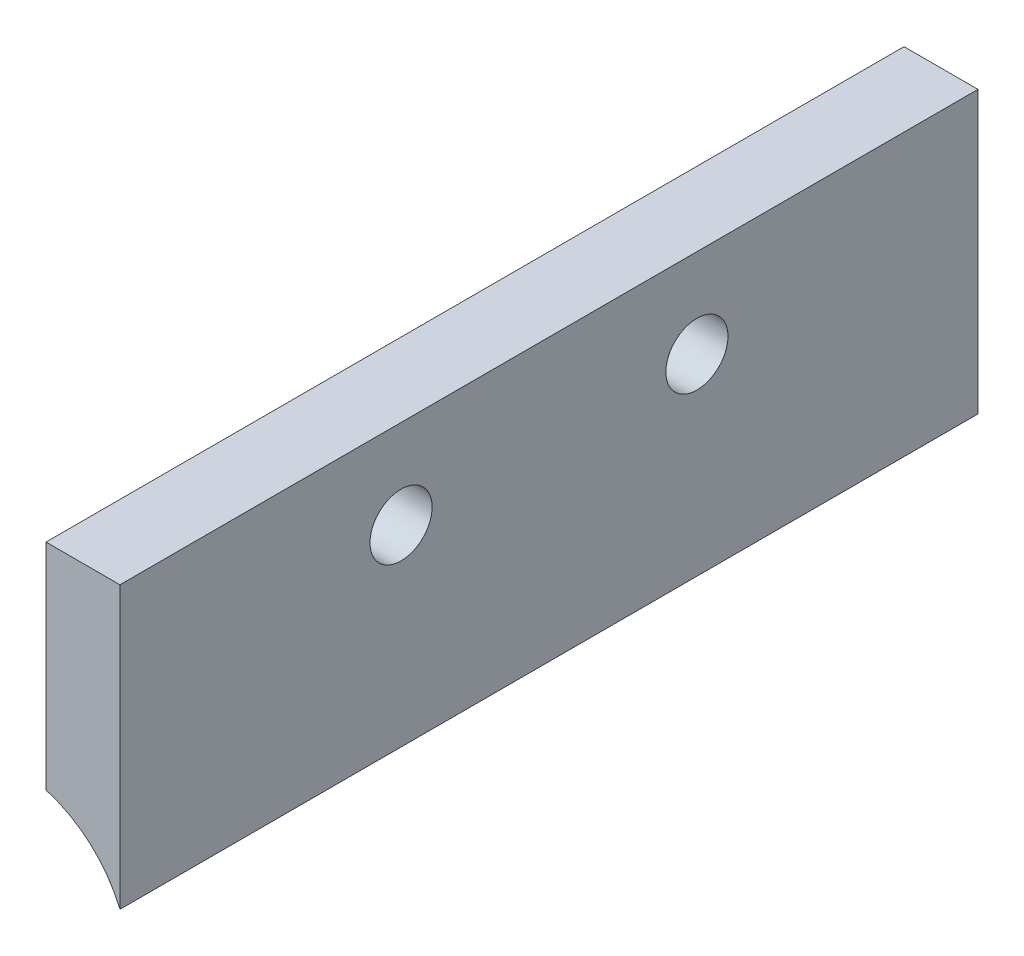
from build123d import *

# Parameters (mm, degrees)
EXTRUDE_1_DEPTH     = 58
SKETCH_2_R          = 2.1
CUT_EXTRUDE_1_DEPTH = 60.630319876


with BuildPart() as part:
    # 草图1 → 凸台-拉伸1 (new body)
    with BuildSketch(Plane.XY):
        with BuildLine():
            Line((-2.777777778, 6.085858586), (2.222222222, 6.085858586))
            Line((2.222222222, 6.085858586), (2.222222222, -12.914141414))
            ThreePointArc((2.222222222, -12.914141414), (0.22943144, -10.106820848), (-2.777777778, -8.430826641))
            Line((-2.777777778, -8.430826641), (-2.777777778, 6.085858586))
        make_face()
    extrude(amount=EXTRUDE_1_DEPTH)

    # 草图2 → 切除-拉伸1 (cut, through all)
    with BuildSketch(Plane.ZY.offset(2.777777778)):
        with Locations(Location((19, 0.085858586, 0), (0, 0, 270))):
            Circle(SKETCH_2_R)
        with Locations(Location((39, 0.085858586, 0), (0, 0, 270))):
            Circle(SKETCH_2_R)
    extrude(amount=-CUT_EXTRUDE_1_DEPTH, mode=Mode.SUBTRACT)


solid = part.part
